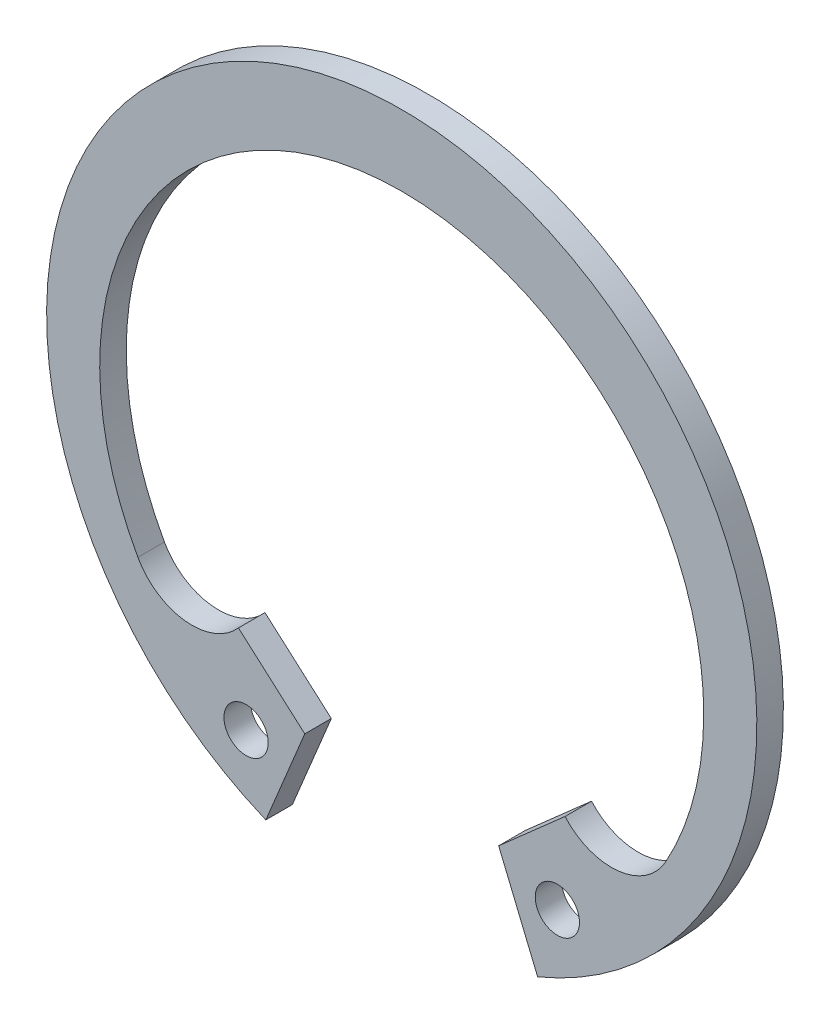
from build123d import *

# Parameters (mm, degrees)
EXTRUDE_947_DEPTH      = 0.6
EXTRUDE_947_DEPTH_BACK = 0.6
SKETCH_1_R             = 1


with BuildPart() as part:
    # 草图1 → Extrude 947 (new, two sides: drawn at the far end of the back side and taken through both)
    with BuildSketch(Plane.XY.offset(-EXTRUDE_947_DEPTH_BACK)):
        with BuildLine():
            Line((-7.380473645, -7.931250769), (-4.381725301, -10.578420647))
            Line((-4.381725301, -10.578420647), (-6.142069089, -14.828266497))
            ThreePointArc((-6.142069089, -14.828266497), (0, 16.05), (6.142069089, -14.828266497))
            Line((6.142069089, -14.828266497), (4.381725301, -10.578420647))
            Line((4.381725301, -10.578420647), (7.380473645, -7.931250769))
            ThreePointArc((7.380473645, -7.931250769), (9.780239262, -8.8620448), (11.925945225, -7.440356203))
            ThreePointArc((11.925945225, -7.440356203), (0, 12.85), (-11.925945225, -7.440356203))
            ThreePointArc((-11.925945225, -7.440356203), (-9.780239262, -8.8620448), (-7.380473645, -7.931250769))
        make_face()
        with Locations((-7.034355028, -11.756183451)):
            Circle(SKETCH_1_R, mode=Mode.SUBTRACT)
        with Locations(Location((7.034355028, -11.756183451, 0), (0, 0, 180))):
            Circle(SKETCH_1_R, mode=Mode.SUBTRACT)
    extrude(amount=EXTRUDE_947_DEPTH + EXTRUDE_947_DEPTH_BACK)


solid = part.part
